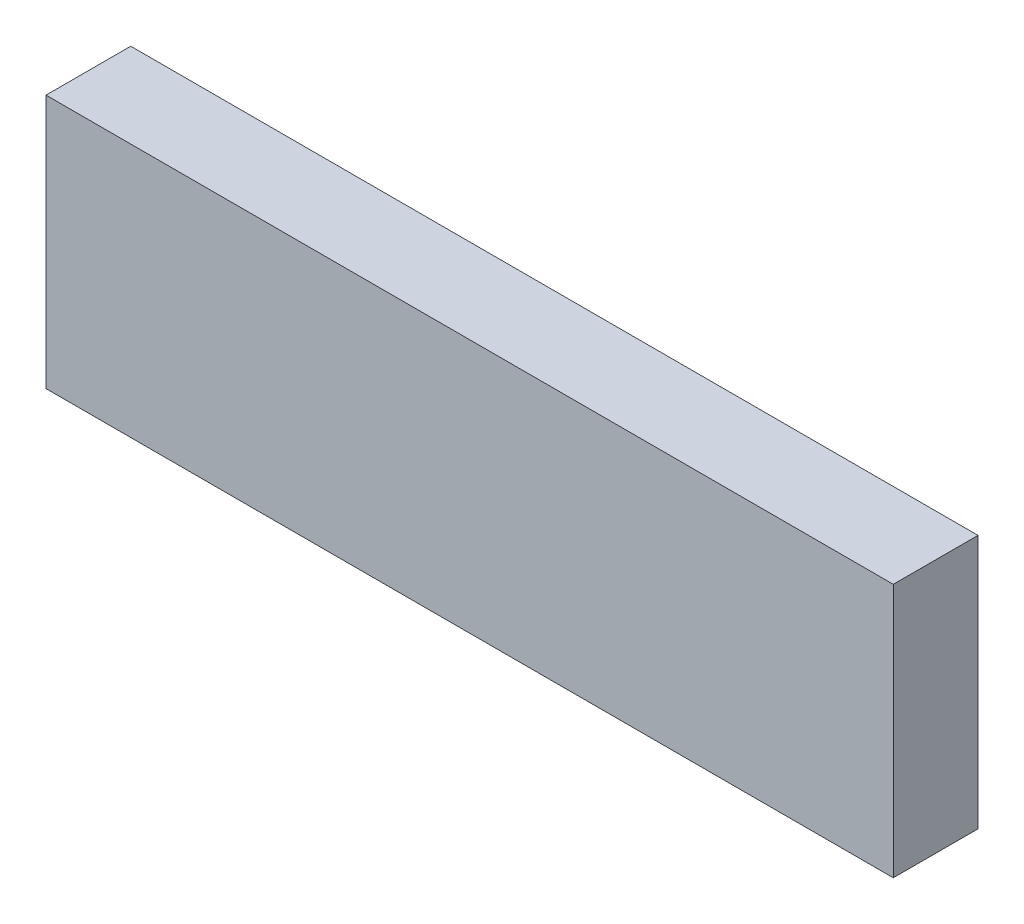
from build123d import *

# Parameters (mm, degrees)
SKETCH1_W           = 200
SKETCH1_H           = 60
BOSS_EXTRUDE1_DEPTH = 20


with BuildPart() as part:
    # Sketch1 → Boss-Extrude1 (new body)
    with BuildSketch(Plane.XY):
        with Locations((100, 30)):
            Rectangle(SKETCH1_W, SKETCH1_H)
    extrude(amount=BOSS_EXTRUDE1_DEPTH)


solid = part.part
